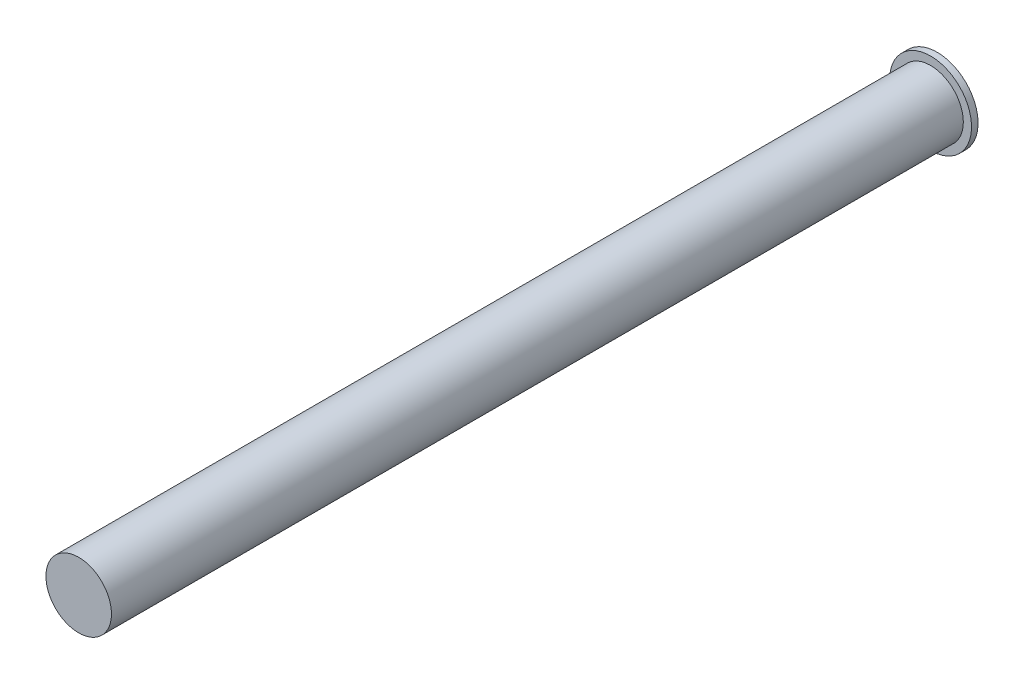
from build123d import *

# Parameters (mm, degrees)
SKETCH_1_R      = 5
EXTRUDE_1_DEPTH = 130
SKETCH_2_R      = 6.25
EXTRUDE_2_DEPTH = 1


with BuildPart() as part:
    # 草图1 → 凸台-拉伸1 (new body)
    with BuildSketch(Plane.XY):
        Circle(SKETCH_1_R)
    extrude(amount=EXTRUDE_1_DEPTH)

    # 草图2 → 凸台-拉伸2 (add)
    with BuildSketch(Plane(origin=(0, 0, 0), x_dir=(-1, 0, 0), z_dir=(0, 0, -1))):
        Circle(SKETCH_2_R)
    extrude(amount=EXTRUDE_2_DEPTH)


solid = part.part
